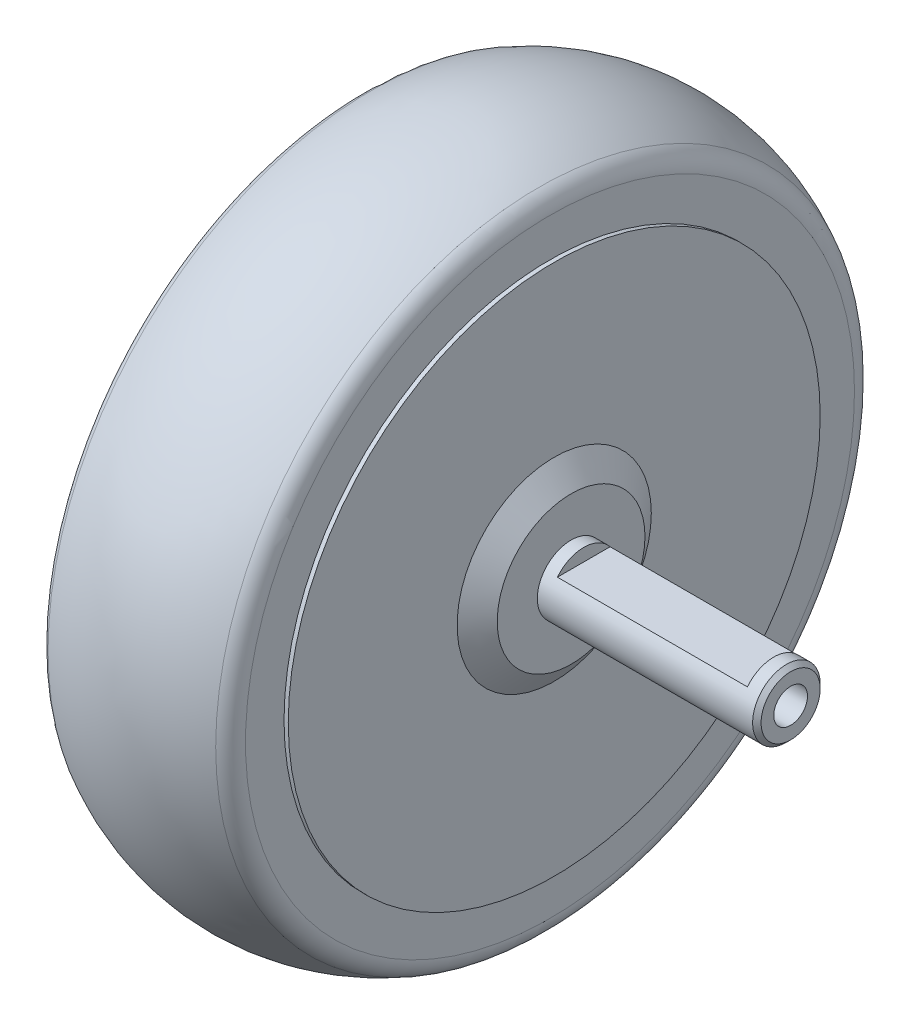
SolidWorks part; units mm, degrees
ref_plane "Front Plane" through (0, 0, 0) normal (0, 0, 1) x (1, 0, 0)
ref_plane "Top Plane" through (0, 0, 0) normal (0, 1, 0) x (1, 0, 0)
ref_plane "Right Plane" through (0, 0, 0) normal (1, 0, 0) x (0, 0, -1)
sketch "Sketch1" plane through (0, 0, 0) normal (0, 0, 1) x (1, 0, 0)
  line L0 (0, 0) -> (-1.6931, 0) construction
  line L1 (0, 9.5943) -> (0, -10.4409) construction
  line L2 (19.5773, 0) -> (19.5773, 50)
  line L3 (19.5773, 50) -> (29.5773, 57)
  line L4 (29.5773, 57) -> (29.5773, 75)
  line L5 (74.5773, 75) -> (74.5773, 63)
  line L6 (74.5773, 63) -> (75.5773, 63)
  line L7 (75.5773, 63) -> (75.5773, 23)
  line L8 (75.5773, 23) -> (79.5773, 17.5)
  line L9 (79.5773, 17.5) -> (79.5773, 8)
  line L10 (79.5773, 8) -> (131.5773, 8)
  line L11 (131.5773, 8) -> (131.5773, 0)
  line L12 (131.5773, 0) -> (19.5773, 0)
  line L13 (52.0773, 81.5) -> (52.0773, 0) construction
  arc A0 (29.5773, 75) -> (74.5773, 75) centre (52.0773, 39.3077) cw
  dimension "D1" = 112
  dimension "D10" = 1
  dimension "D19" = 42.1923
  dimension "D21" = 42.1923
  dimension "D2" = 0
  dimension "D3" = 10
  dimension "D4" = 18
  dimension "D5" = 45
  dimension "D6" = 46
  dimension "D7" = 35
  dimension "D8" = 8
  dimension "D9" = 40
  dimension "D11" = 45.3982
  dimension "D12" = 50
  dimension "D13" = 81.5
  dimension "D14" = 45
  dimension "D15" = 56
  dimension "D16" = 52
  dimension "D17" = 4
  dimension "D18" = 12
  dimension "D20" = 5.5
revolve "Revolve1" add sketch "Sketch1" angle 360 about L0
fillet "Fillet1" radius 5 2 edges at (29.5773, 0, -75) (74.5773, 0, -75)
sketch "Sketch2" plane through (19.5773, 0, 0) normal (-1, 0, 0) x (0, 0, 1)
  line L36 (-22.4948, 6.2599) -> (-42.8978, 13.0034)
  line L37 (-42.8978, -13.0034) -> (-22.4948, -6.2599)
  line L38 (-16.6686, -16.3511) -> (-32.7102, -30.6488)
  line L39 (-10.1876, -43.6523) -> (-5.8262, -22.611)
  line L40 (5.8262, -22.611) -> (10.1876, -43.6523)
  line L41 (32.7102, -30.6488) -> (16.6686, -16.3511)
  line L42 (22.4948, -6.2599) -> (42.8978, -13.0034)
  line L43 (42.8978, 13.0034) -> (22.4948, 6.2599)
  line L44 (16.6686, 16.3511) -> (32.7102, 30.6488)
  line L45 (10.1876, 43.6523) -> (5.8262, 22.611)
  line L46 (-5.8262, 22.611) -> (-10.1876, 43.6523)
  line L47 (-32.7102, 30.6488) -> (-16.6686, 16.3511)
  arc A72 (-22.4948, 6.2599) -> (-16.6686, 16.3511) centre (-20.6275, 11.9093) ccw
  arc A73 (-42.8978, 13.0034) -> (-46.7618, 10.832) centre (-43.8392, 10.155) ccw
  arc A74 (-46.7618, 10.832) -> (-46.7618, -10.832) centre (0, 0) ccw
  arc A75 (-46.7618, -10.832) -> (-42.8978, -13.0034) centre (-43.8392, -10.155) ccw
  arc A76 (-16.6686, -16.3511) -> (-22.4948, -6.2599) centre (-20.6275, -11.9093) ccw
  arc A77 (-32.7102, -30.6488) -> (-32.7617, -35.0809) centre (-30.7141, -32.8884) ccw
  arc A78 (-32.7617, -35.0809) -> (-14.0001, -45.9129) centre (0, 0) ccw
  arc A79 (-14.0001, -45.9129) -> (-10.1876, -43.6523) centre (-13.1251, -43.0434) ccw
  arc A80 (5.8262, -22.611) -> (-5.8262, -22.611) centre (0, -23.8186) ccw
  arc A81 (10.1876, -43.6523) -> (14.0001, -45.9129) centre (13.1251, -43.0434) ccw
  arc A82 (14.0001, -45.9129) -> (32.7617, -35.0809) centre (0, 0) ccw
  arc A83 (32.7617, -35.0809) -> (32.7102, -30.6488) centre (30.7141, -32.8884) ccw
  arc A84 (22.4948, -6.2599) -> (16.6686, -16.3511) centre (20.6275, -11.9093) ccw
  arc A85 (42.8978, -13.0034) -> (46.7618, -10.832) centre (43.8392, -10.155) ccw
  arc A86 (46.7618, -10.832) -> (46.7618, 10.832) centre (0, 0) ccw
  arc A87 (46.7618, 10.832) -> (42.8978, 13.0034) centre (43.8392, 10.155) ccw
  arc A88 (16.6686, 16.3511) -> (22.4948, 6.2599) centre (20.6275, 11.9093) ccw
  arc A89 (32.7102, 30.6488) -> (32.7617, 35.0809) centre (30.7141, 32.8884) ccw
  arc A90 (32.7617, 35.0809) -> (14.0001, 45.9129) centre (0, 0) ccw
  arc A91 (14.0001, 45.9129) -> (10.1876, 43.6523) centre (13.1251, 43.0434) ccw
  arc A92 (-5.8262, 22.611) -> (5.8262, 22.611) centre (0, 23.8186) ccw
  arc A93 (-10.1876, 43.6523) -> (-14.0001, 45.9129) centre (-13.1251, 43.0434) ccw
  arc A94 (-14.0001, 45.9129) -> (-32.7617, 35.0809) centre (0, 0) ccw
  arc A95 (-32.7617, 35.0809) -> (-32.7102, 30.6488) centre (-30.7141, 32.8884) ccw
sketch "Sketch3" plane through (131.5773, 0, 0) normal (1, 0, 0) x (0, 0, -1)
  line L1 (-6.245, 5) -> (6.245, 5)
  line L2 (0, 8) -> (0, -8) construction
  circle A1 centre (0, 0) radius 8 construction
  arc A2 (6.245, 5) -> (-6.245, 5) centre (0, 0) ccw
  circle A3 centre (0, 0) radius 8 construction
  dimension "D1" = 16
  dimension "D2" = 13
  dimension "D3" = 3
  dimension "D4" = 13
extrude "Cut-Extrude2" cut sketch "Sketch3" against normal blind 45 from offset 4 offset against normal yes
chamfer "Chamfer1" distance 1 angle 45 1 edges at (131.5773, 0, -8)
sketch "Sketch4" plane through (131.5773, 0, 0) normal (1, 0, 0) x (0, 0, -1)
  circle A0 centre (0, 0) radius 4
  dimension "D1" = 8
extrude "Cut-Extrude3" cut sketch "Sketch4" against normal blind 50
ref_plane "Plane1" through (0, 81.5, 0) normal (0, 1, 0) x (1, 0, 0)
sketch "Sketch6" plane through (0, 81.5, 0) normal (0, 1, 0) x (1, 0, 0)
  line L0 (131.5773, 0) -> (29.5773, 0) construction
  line L1 (131.5773, -7) -> (131.5773, 7) construction
  line L2 (29.5773, 57) -> (29.5773, -57) construction
  line L3 (29.5773, 0) -> (29.5773, 4.4485)
  line L4 (74.5773, 5.1834) -> (74.5773, 1.995)
  line L5 (74.5773, -63) -> (74.5773, 63) construction
  line L6 (29.5773, 4.4485) -> (29.5773, 3.1793)
  line L7 (29.5773, 3.1793) -> (30.4655, 3.2397)
  spline S0 degree 3 poles (29.5773, 4.4485) (31.9685, 6.2053) (40.5925, 7.9461) (50.4587, -1.971) (63.6711, -6.4616) (70.3225, -3.6454) (74.5773, 5.1834) knots 0.06645 0.06645 0.06645 0.06645 0.203596 0.563424 0.638525 0.954598 0.954598 0.954598 0.954598
  spline S1 degree 1 poles (30.4655, 3.2397) (75.9286, 4.5322) knots 0 0 1 1 construction
  spline S2 degree 3 poles (30.4655, 3.2397) (30.6724, 3.3917) (31.1067, 3.6878) (31.9365, 4.166) (32.959, 4.6038) (34.1616, 4.8985) (35.77, 5.0269) (37.8443, 4.7315) (40.4852, 3.7366) (43.2362, 2.2385) (47.0117, -0.1866) (51.8761, -3.5519) (57.0643, -6.0121) (61.369, -6.7013) (64.6285, -6.4441) (67.8121, -5.2623) (70.2945, -3.4563) (72.1512, -1.5048) (73.3681, 0.0746) (74.2158, 1.3816) (74.8352, 2.4309) (75.3388, 3.3439) (75.7385, 4.1377) (75.9286, 4.5322) knots 0.06645 0.06645 0.06645 0.06645 0.080328 0.094205 0.12196 0.149714 0.177469 0.232978 0.288487 0.343997 0.399506 0.510524 0.621543 0.677052 0.732561 0.78807 0.84358 0.871334 0.899089 0.91993 0.926869 0.940721 0.954598 0.954598 0.954598 0.954598 only from (30.4655, 3.2397) to (74.5773, 1.995)
  dimension "D1" = 1.5
